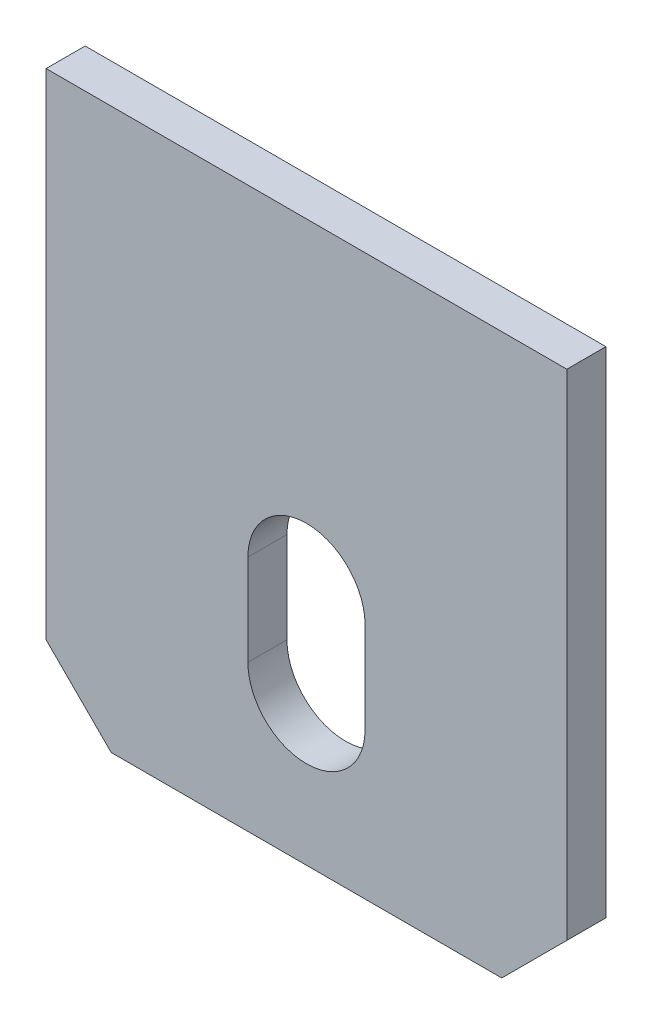
SolidWorks part; units mm, degrees
ref_plane "Front Plane" through (0, 0, 0) normal (0, 0, 1) x (1, 0, 0)
ref_plane "Top Plane" through (0, 0, 0) normal (0, 1, 0) x (1, 0, 0)
ref_plane "Right Plane" through (0, 0, 0) normal (1, 0, 0) x (0, 0, -1)
sketch "Sketch1" plane through (0, 0, 0) normal (0, 0, 1) x (1, 0, 0)
  line L0 (213.5854, 213.4953) -> (253.5854, 213.4953)
  line L1 (253.5854, 213.4953) -> (253.5854, 175.4953)
  line L2 (248.5854, 170.4953) -> (253.5854, 175.4953)
  line L3 (248.5854, 170.4953) -> (218.5854, 170.4953)
  line L4 (213.5854, 175.4953) -> (213.5854, 213.4953)
  line L5 (218.5854, 170.4953) -> (213.5854, 175.4953)
  line L6 (229.0854, 181.7453) -> (229.0854, 188.7453)
  line L7 (238.0854, 181.7453) -> (238.0854, 188.7453)
  arc A0 (229.0854, 181.7453) -> (238.0854, 181.7453) centre (233.5854, 181.7453) ccw
  arc A1 (238.0854, 188.7453) -> (229.0854, 188.7453) centre (233.5854, 188.7453) ccw
extrude "Boss-Extrude1" add sketch "Sketch1" along normal blind 3
